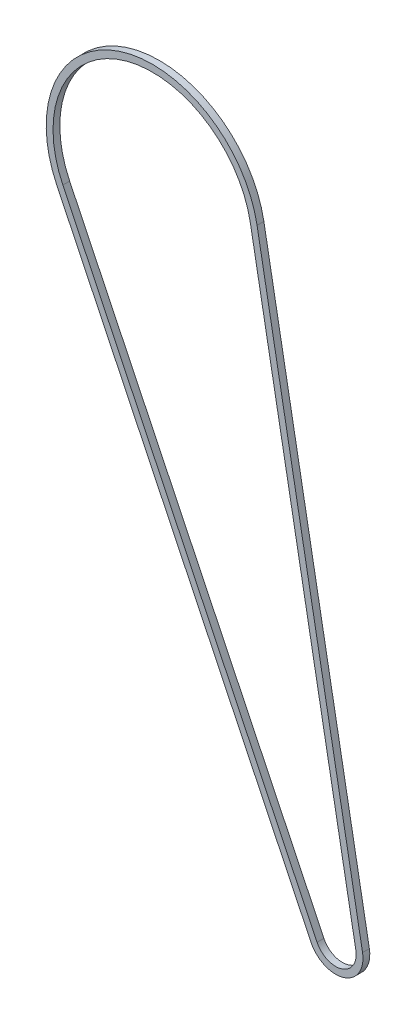
from build123d import *

# Parameters (mm, degrees)
THIN_WALL_EXTRUDE1_DEPTH = 10


with BuildPart() as part:
    # Sketch1 → Thin-wall extrude1 (new body)
    with BuildSketch(Plane.XY):
        with BuildLine():
            Line((153.510023011, 111.669421793), (308.383834576, -735.55582317))
            ThreePointArc((308.383834576, -735.55582317), (281.282561977, -781.001122311), (232.629670707, -760.200873238))
            Line((232.629670707, -760.200873238), (-140.636470033, 15.974945367))
            ThreePointArc((-140.636470033, 15.974945367), (-48.278259042, 232.005723732), (153.510023011, 111.669421793))
        make_face()
        with BuildLine():
            Line((143.673030314, 109.87120749), (298.546841879, -737.354037473))
            ThreePointArc((298.546841879, -737.354037473), (278.18886899, -771.491702575), (241.641720223, -755.866941592))
            Line((241.641720223, -755.866941592), (-131.624420517, 20.308877014))
            ThreePointArc((-131.624420517, 20.308877014), (-45.184566055, 222.496303997), (143.673030314, 109.87120749))
        make_face(mode=Mode.SUBTRACT)
    extrude(amount=THIN_WALL_EXTRUDE1_DEPTH)


solid = part.part
